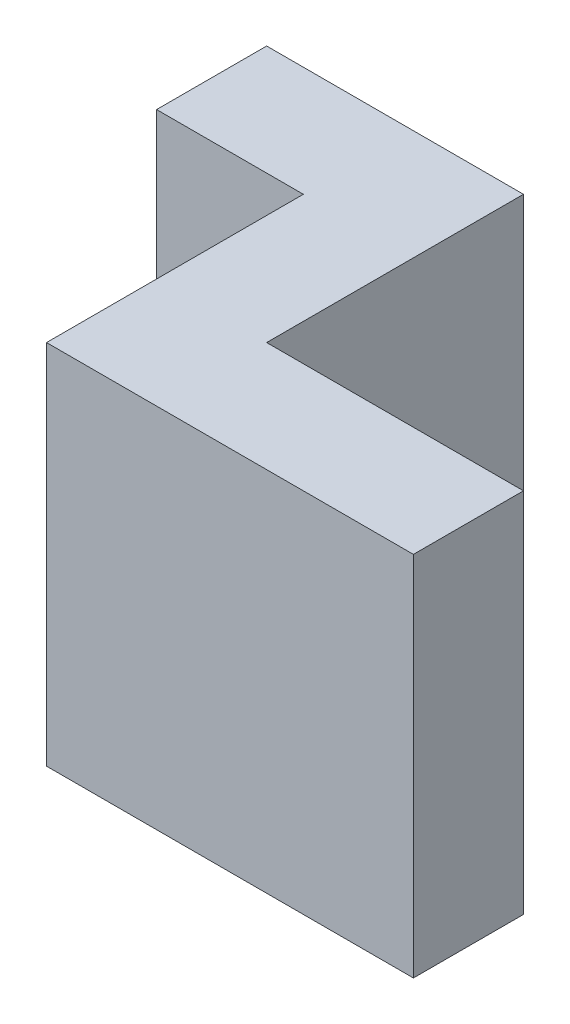
SolidWorks part; units mm, degrees
ref_plane "Front Plane" through (0, 0, 0) normal (0, 0, 1) x (1, 0, 0)
ref_plane "Top Plane" through (0, 0, 0) normal (0, 1, 0) x (1, 0, 0)
ref_plane "Right Plane" through (0, 0, 0) normal (1, 0, 0) x (0, 0, -1)
sketch "Sketch1" plane through (0, 0, 0) normal (0, 1, 0) x (1, 0, 0)
  line L0 (0, 0) -> (4, 0)
  line L1 (4, 0) -> (4, -7)
  line L2 (4, -7) -> (14, -7)
  line L3 (0, 3) -> (7, 3)
  line L4 (7, 3) -> (7, -4)
  line L5 (7, -4) -> (14, -4)
  line L6 (0, 3) -> (0, 0)
  line L7 (14, -4) -> (14, -7)
  dimension "D1" = 7
  dimension "D2" = 4
  dimension "D3" = 10
  dimension "D4" = 3
extrude "Boss-Extrude1" add sketch "Sketch1" along normal blind 10
